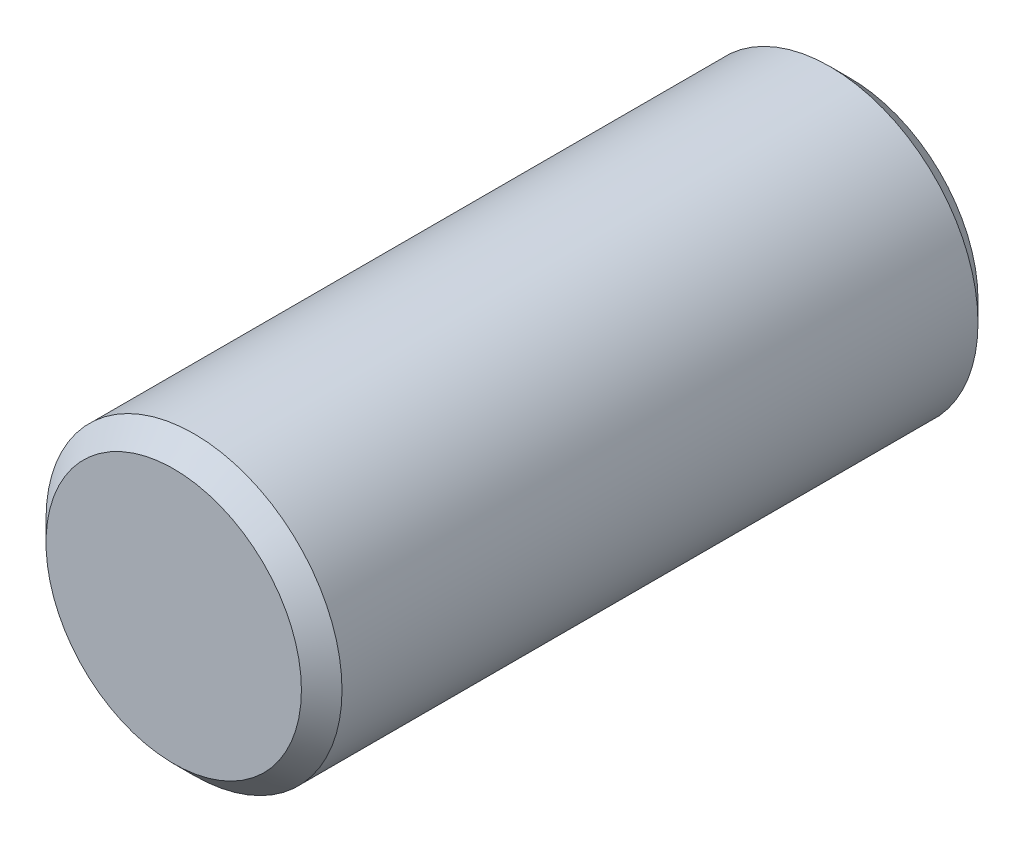
from build123d import *

# Parameters (mm, degrees)
SKETCH1_R      = 11.1125
EXTRUDE1_DEPTH = 25.4
CHAMFER1_SIZE  = 1.524


with BuildPart() as part:
    # Sketch1 → Extrude1 (new, symmetric)
    with BuildSketch(Plane.XY):
        Circle(SKETCH1_R)
    extrude(amount=EXTRUDE1_DEPTH, both=True)

    # Chamfer1
    chamfer1_edges = [part.edges().sort_by_distance(p)[0] for p in [
        (-11.1125, 0, -25.4),
        (-11.1125, 0, 25.4),
    ]]
    chamfer(chamfer1_edges, length=CHAMFER1_SIZE)


solid = part.part
